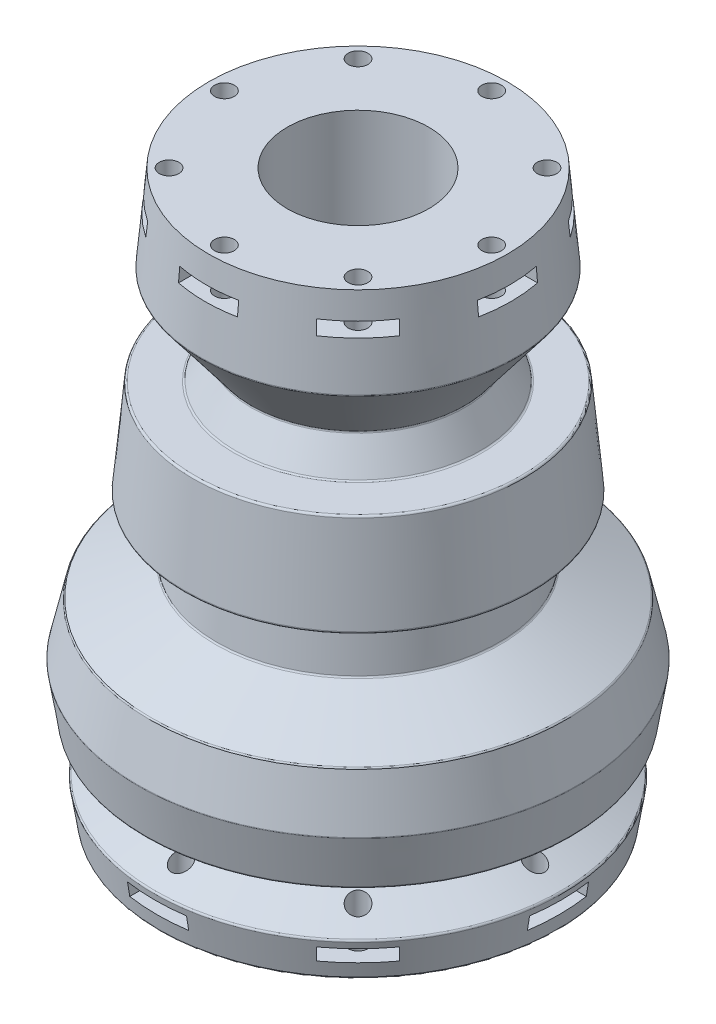
from build123d import *

# Parameters (mm, degrees)
CUT_EXTRUDE_START        = -10
SKETCH_2_W               = 15
SKETCH_2_H               = 26
CUT_EXTRUDE_1_DEPTH      = 3.5
SKETCH_3_R               = 2.5
CUT_EXTRUDE_2_DEPTH      = 15
SKETCH_4_R               = 2.5
CUT_EXTRUDE_3_DEPTH      = 15
CUT_EXTRUDE_START_2      = -4
SKETCH_5_W               = 15
SKETCH_5_H               = 20
CUT_EXTRUDE_4_DEPTH      = 3.5
PATTERN_CIRCULAR_1_COUNT = 8
EXTRUDE_START            = 15
SKETCH_6_R               = 25
SKETCH_6_R_2             = 18
EXTRUDE_1_DEPTH          = 15
SKETCH_7_R               = 2.75
CUT_EXTRUDE_5_DEPTH      = 50
CUT_EXTRUDE_START_3      = -24
SKETCH_8_R               = 5
CUT_EXTRUDE_6_DEPTH      = 50
PATTERN_CIRCULAR_2_COUNT = 4
FILLET_1_R               = 0.5


with BuildPart() as part:
    # 草图1 → 旋转1 (revolve)
    with BuildSketch(Plane.XY, mode=Mode.PRIVATE) as revolve_1_sk:
        Polygon((38, 0), (18, 0), (18, -143), (50.5, -143), (52, -133.6), (37.3, -126.6), (38.5, -120.6), (54, -120.6), (56, -108.1), (53, -94.8), (36, -86.8), (34.5, -71.5), (44.3, -71.5), (42, -47), (31.3, -47), (27, -39), (40, -22), align=None)
    revolve(revolve_1_sk.sketch.rotate(Axis((0, 0, 0), (0, -1, 0)), 90), axis=Axis((0, 0, 0), (0, -1, 0)))

    # 草图2 → 切除-拉伸1 (cut)
    with BuildSketch(Plane(origin=(0, 0, 0), x_dir=(1, 0, 0), z_dir=(0, 1, 0)).offset(CUT_EXTRUDE_START)):
        with Locations((0, -38)):
            Rectangle(SKETCH_2_W, SKETCH_2_H)
    cut_extrude_1 = extrude(amount=CUT_EXTRUDE_1_DEPTH, mode=Mode.SUBTRACT)

    # 草图3 → 切除-拉伸2 (cut)
    with BuildSketch(Plane(origin=(0, 0, 0), x_dir=(1, 0, 0), z_dir=(0, 1, 0))):
        with Locations(Location((0, -34, 0), (0, 0, 270))):
            Circle(SKETCH_3_R)
    cut_extrude_2 = extrude(amount=-CUT_EXTRUDE_2_DEPTH, mode=Mode.SUBTRACT)

    # 草图4 → 切除-拉伸3 (cut)
    with BuildSketch(Plane.XZ.offset(143)):
        with Locations(Location((0, 45, 0), (0, 0, 270))):
            Circle(SKETCH_4_R)
    cut_extrude_3 = extrude(amount=-CUT_EXTRUDE_3_DEPTH, mode=Mode.SUBTRACT)

    # 草图5 → 切除-拉伸4 (cut)
    with BuildSketch(Plane.XZ.offset(143).offset(CUT_EXTRUDE_START_2)):
        with Locations((0, 45)):
            Rectangle(SKETCH_5_W, SKETCH_5_H)
    cut_extrude_4 = extrude(amount=-CUT_EXTRUDE_4_DEPTH, mode=Mode.SUBTRACT)

    # 阵列(圆周)1: 切除-拉伸1, 切除-拉伸2, 切除-拉伸3, 切除-拉伸4 ×8 about axis
    pattern_circular_1_axis = Axis((0, 0, 0), (0, 1, 0))
    add([cut_extrude_1.rotate(pattern_circular_1_axis, i * 360 / PATTERN_CIRCULAR_1_COUNT) for i in range(1, PATTERN_CIRCULAR_1_COUNT)], mode=Mode.SUBTRACT)
    add([cut_extrude_2.rotate(pattern_circular_1_axis, i * 360 / PATTERN_CIRCULAR_1_COUNT) for i in range(1, PATTERN_CIRCULAR_1_COUNT)], mode=Mode.SUBTRACT)
    add([cut_extrude_3.rotate(pattern_circular_1_axis, i * 360 / PATTERN_CIRCULAR_1_COUNT) for i in range(1, PATTERN_CIRCULAR_1_COUNT)], mode=Mode.SUBTRACT)
    add([cut_extrude_4.rotate(pattern_circular_1_axis, i * 360 / PATTERN_CIRCULAR_1_COUNT) for i in range(1, PATTERN_CIRCULAR_1_COUNT)], mode=Mode.SUBTRACT)

    # 草图6 → 凸台-拉伸1 (add)
    with BuildSketch(Plane.XZ.offset(143).offset(EXTRUDE_START)):
        with Locations(Location((0, 0, 0), (0, 0, 90))):
            Circle(SKETCH_6_R)
        with Locations(Location((0, 0, 0), (0, 0, 90))):
            Circle(SKETCH_6_R_2, mode=Mode.SUBTRACT)
    extrude(amount=-EXTRUDE_1_DEPTH)

    # 草图7 → 切除-拉伸5 (cut)
    with BuildSketch(Plane.XY):
        with Locations((0, -151)):
            Circle(SKETCH_7_R)
    cut_extrude_5 = extrude(amount=-CUT_EXTRUDE_5_DEPTH, mode=Mode.SUBTRACT)

    # 草图8 → 切除-拉伸6 (cut)
    with BuildSketch(Plane.XY.offset(CUT_EXTRUDE_START_3)):
        with Locations((0, -151)):
            Circle(SKETCH_8_R)
    cut_extrude_6 = extrude(amount=-CUT_EXTRUDE_6_DEPTH, mode=Mode.SUBTRACT)

    # 阵列(圆周)2: 切除-拉伸5, 切除-拉伸6 ×4 about axis
    pattern_circular_2_axis = Axis((0, 0, 0), (0, 1, 0))
    add([cut_extrude_5.rotate(pattern_circular_2_axis, i * 360 / PATTERN_CIRCULAR_2_COUNT) for i in range(1, PATTERN_CIRCULAR_2_COUNT)], mode=Mode.SUBTRACT)
    add([cut_extrude_6.rotate(pattern_circular_2_axis, i * 360 / PATTERN_CIRCULAR_2_COUNT) for i in range(1, PATTERN_CIRCULAR_2_COUNT)], mode=Mode.SUBTRACT)

    # 圆角1
    fillet_1_edges = [part.edges().sort_by_distance(p)[0] for p in [
        (0, -22, -40),
        (0, -39, -27),
        (0, -47, -31.3),
        (0, -47, -42),
        (0, -71.5, -44.3),
        (0, -71.5, -34.5),
        (0, -86.8, -36),
        (0, -94.8, -53),
        (0, -108.1, -56),
        (0, -120.6, -54),
        (0, -120.6, -38.5),
        (0, -126.6, -37.3),
        (0, -133.6, -52),
        (0, -143, -50.5),
        (0, -143, -25),
    ]]
    fillet(fillet_1_edges, radius=FILLET_1_R)


solid = part.part
